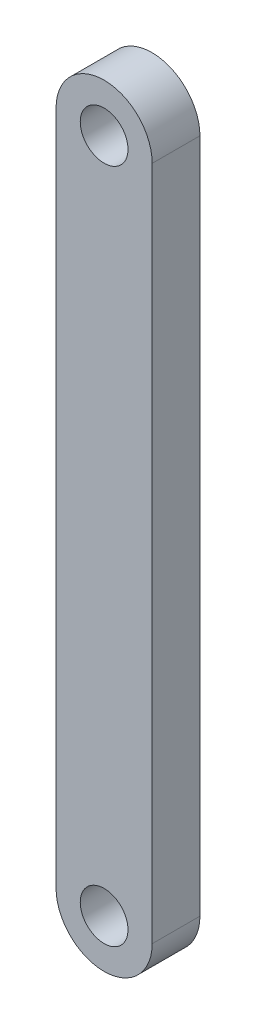
SolidWorks part; units mm, degrees
ref_plane "Front Plane" through (0, 0, 0) normal (0, 0, 1) x (1, 0, 0)
ref_plane "Top Plane" through (0, 0, 0) normal (0, 1, 0) x (1, 0, 0)
ref_plane "Right Plane" through (0, 0, 0) normal (1, 0, 0) x (0, 0, -1)
sketch "Sketch1" plane through (0, 0, 0) normal (0, 0, 1) x (1, 0, 0)
  line L0 (0, 0) -> (0, 45) construction
  line L1 (-3.2, 0) -> (-3.2, 45)
  line L2 (3.2, 0) -> (3.2, 45)
  arc A0 (-3.2, 0) -> (3.2, 0) centre (0, 0) ccw
  arc A1 (3.2, 45) -> (-3.2, 45) centre (0, 45) ccw
  circle A2 centre (0, 0) radius 1.59
  circle A3 centre (0, 45) radius 1.59
  point P3 (0, 22.5)
  dimension "D1" = 3.18
  dimension "D2" = 3.18
  dimension "D3" = 3.2
  dimension "D4" = 45
extrude "Boss-Extrude1" add sketch "Sketch1" along normal blind 3.18
scale "Scale ratio 1" scale about origin uniform scaling yes scale factor 1.3
